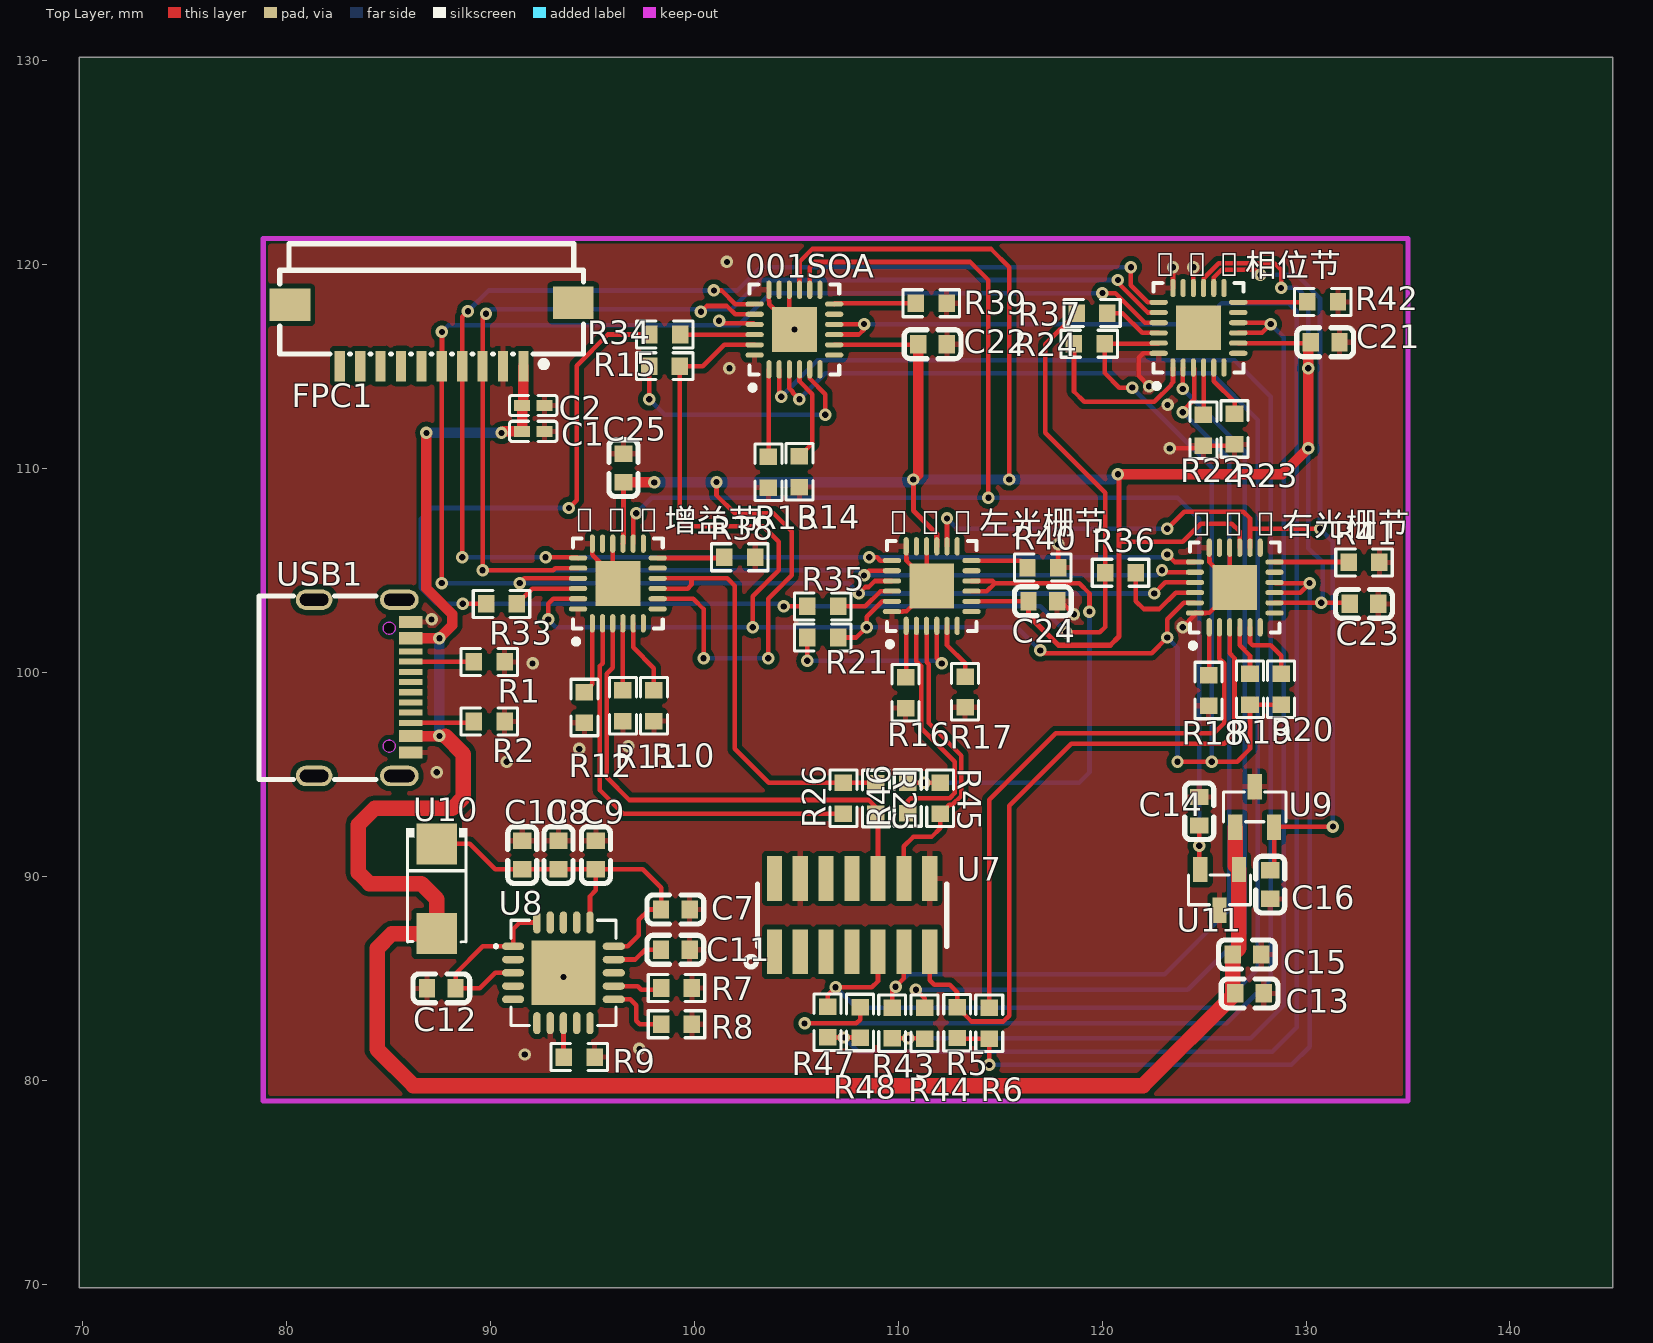
[diagram p0: Top Layer view]
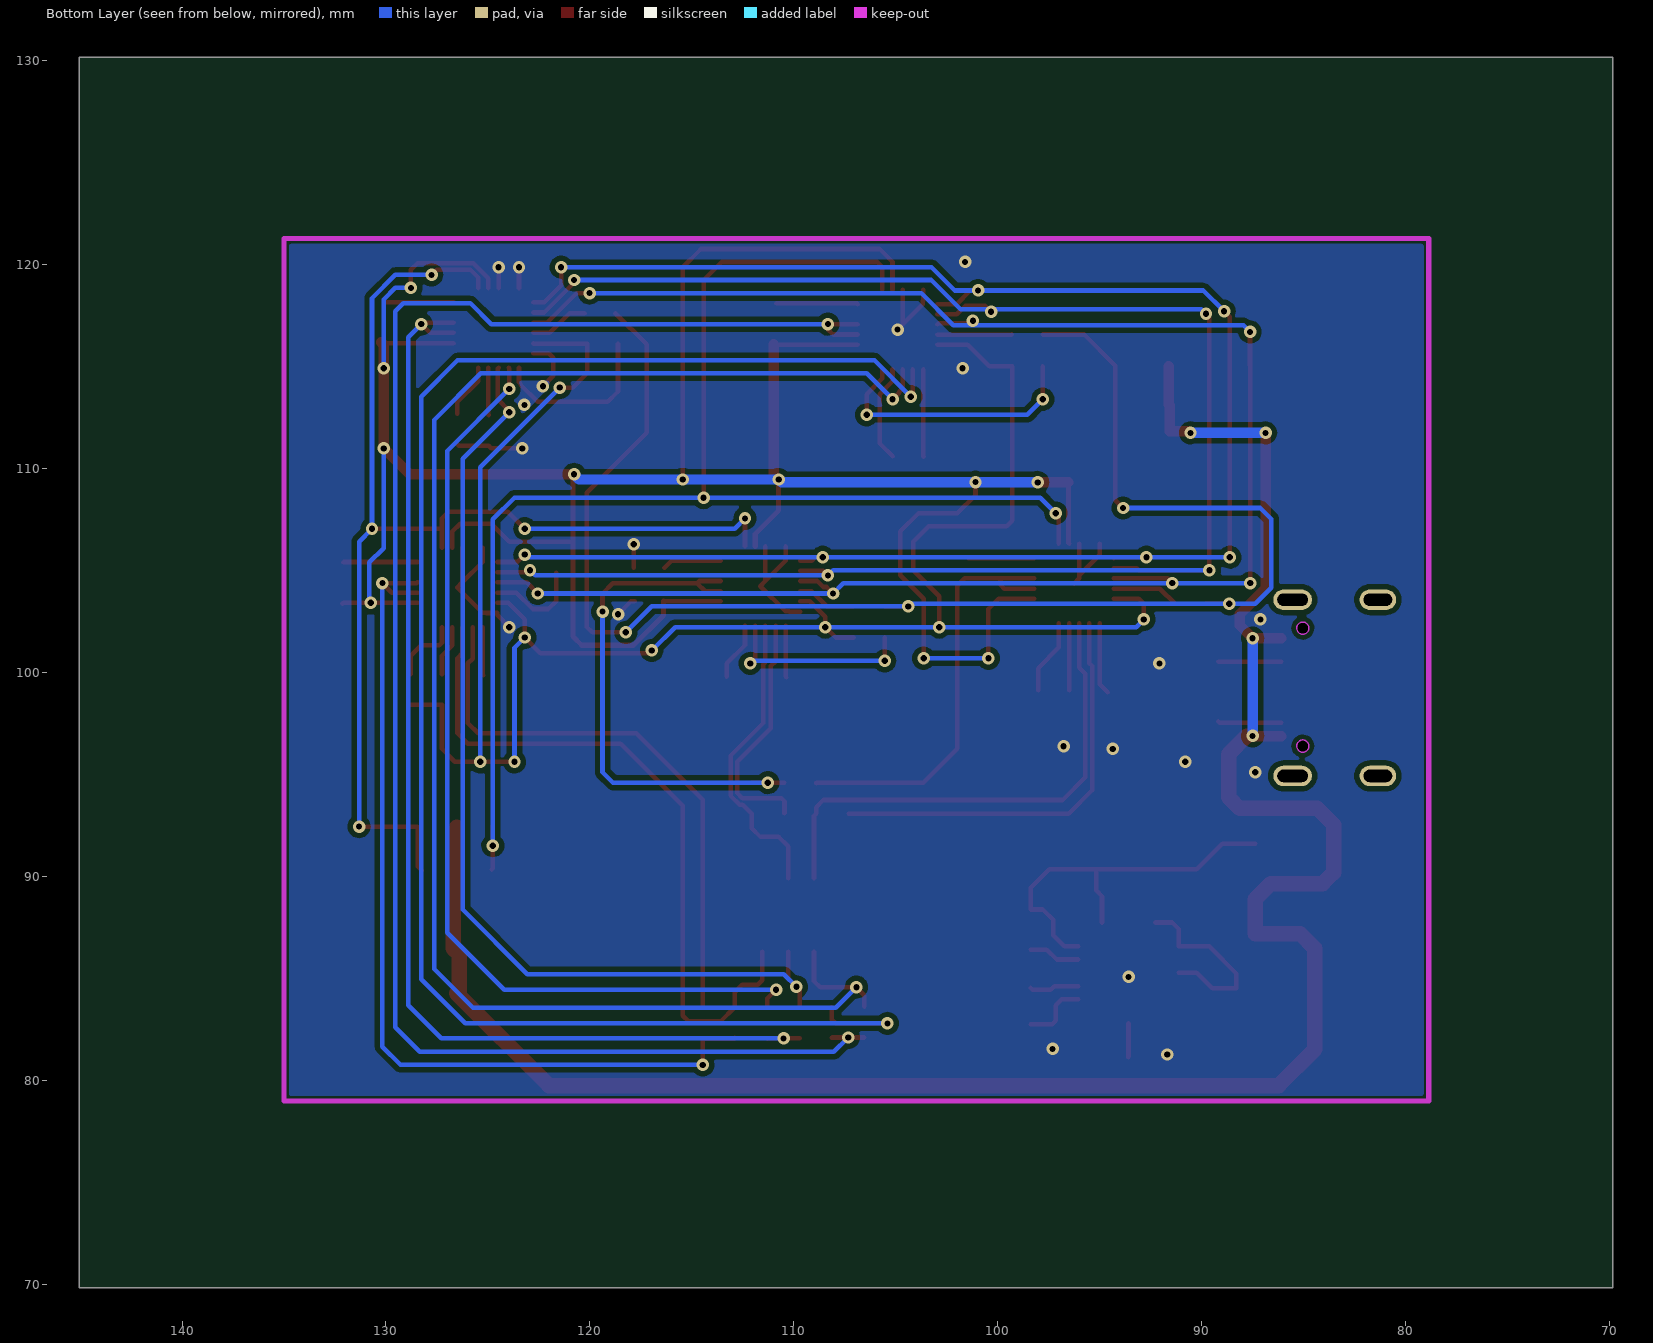
[diagram p1: Bottom Layer view, seen from below]
# Altium PCB MISC49874.pcbdoc
Units mm, origin at the board's own origin, x right, y up, seen from the top; angles counter-clockwise.
Board outline 75.18 x 60.32 mm, 2 copper layers (Top Layer, Bottom Layer), stack 1.58 mm thick; 69 components, 60 nets, 310 pads, 95 vias.

## Layer stack, top to bottom
Top Solder Mask Layer: solder mask 0.01, Dk 3.3
Top Layer: signal copper 0.035
Dielectric1: surface 1.51, FR4, Dk 4.5
Bottom Layer: signal copper 0.035
Bottom Solder Mask Layer: solder mask 0.01, Dk 3.3

## Board outline
145.034,69.85 69.85,69.85 69.85,130.175 145.034,130.175

## Design rules (kind name [scope] priority, off if disabled: settings)
BoardOutlineClearance copperThickness2oz_1 [All] p2 off: genericclearance=0.203 ignorepadtopadclearanceinfootprint=FALSE except(0: Arc-SplitContinuation Track-SplitContinuation SMDPad-SplitContinuation THPad-SplitContinuation Via-SplitContinuation Fill-SplitContinuation Region-SplitContinuation Poly-SplitContinuation Text-SplitContinuation Hole-SplitContinuation; 0.152: Arc-CutoutEdge SMDPad-CutoutEdge THPad-CutoutEdge Via-CutoutEdge Fill-CutoutEdge Region-CutoutEdge Text-CutoutEdge; 0.176: Hole-OutlineEdge Hole-CutoutEdge; 0.254: Poly-OutlineEdge Poly-CutoutEdge; 0.3: Arc-OutlineEdge Track-OutlineEdge SMDPad-OutlineEdge THPad-OutlineEdge Via-OutlineEdge Fill-OutlineEdge Region-OutlineEdge Text-OutlineEdge Track-CutoutEdge)
BoardOutlineClearance copperThickness1oz_1 [All] p4: genericclearance=0.102 ignorepadtopadclearanceinfootprint=FALSE except(0: Arc-SplitContinuation Track-SplitContinuation SMDPad-SplitContinuation THPad-SplitContinuation Via-SplitContinuation Fill-SplitContinuation Region-SplitContinuation Poly-SplitContinuation Text-SplitContinuation Hole-SplitContinuation; 0.152: SMDPad-CutoutEdge THPad-CutoutEdge Via-CutoutEdge Fill-CutoutEdge Region-CutoutEdge Text-CutoutEdge; 0.176: Hole-OutlineEdge Hole-CutoutEdge; 0.254: Poly-OutlineEdge Poly-CutoutEdge; 0.3: Arc-OutlineEdge Track-OutlineEdge SMDPad-OutlineEdge THPad-OutlineEdge Via-OutlineEdge Fill-OutlineEdge Region-OutlineEdge Text-OutlineEdge Arc-CutoutEdge Track-CutoutEdge)
Clearance copperThickness2oz [All] p1 off: gap=0.203 ignorepadtopadclearanceinfootprint=FALSE except(0.152: SMDPad-Track SMDPad-SMDPad THPad-Track SMDPad-THPad THPad-THPad Track-Via SMDPad-Via THPad-Via Via-Via Fill-Track Region-Track Fill-SMDPad Region-SMDPad Fill-THPad Region-THPad Fill-Via Region-Via Fill-Fill Fill-Region Region-Region Arc-Track Arc-SMDPad Arc-THPad Arc-Via Fill-Arc Region-Arc Arc-Arc Text-Track SMDPad-Text Text-THPad Text-Via Fill-Text Region-Text Arc-Text Text-Text; 0.176: Hole-Track Hole-SMDPad Hole-THPad Hole-Via Fill-Hole Region-Hole Hole-Arc Hole-Text; 0.254: Poly-Track Poly-SMDPad Poly-THPad Poly-Via Poly-Fill Poly-Region Poly-Poly Poly-Arc Poly-Text Poly-Hole)
Clearance copperThickness1oz [All] p3: gap=0.102 ignorepadtopadclearanceinfootprint=FALSE except(0.152: SMDPad-Track SMDPad-SMDPad THPad-Track SMDPad-THPad THPad-THPad Track-Via SMDPad-Via THPad-Via Via-Via Fill-Track Region-Track Fill-SMDPad Region-SMDPad Fill-THPad Region-THPad Fill-Via Region-Via Fill-Fill Fill-Region Region-Region Arc-Track Arc-SMDPad Arc-THPad Arc-Via Fill-Arc Region-Arc Arc-Arc Text-Track SMDPad-Text Text-THPad Text-Via Fill-Text Region-Text Arc-Text Text-Text; 0.176: Hole-Track Hole-SMDPad Hole-THPad Hole-Via Fill-Hole Region-Hole Hole-Arc Hole-Text; 0.254: Poly-Track Poly-SMDPad Poly-THPad Poly-Via Poly-Fill Poly-Region Poly-Poly Poly-Arc Poly-Text Poly-Hole)
DiffPairsRouting differentialPair [All] p1: maxlimit=0.152 minlimit=0.152 mostfreqgap=0.152 toplayer_minwidth=0.127 toplayer_prefwidth=0.254 toplayer_maxwidth=2.54 toplayer_mingap=0.152 toplayer_prefgap=0.152 toplayer_maxgap=0.152 bottomlayer_minwidth=0.127 bottomlayer_prefwidth=0.254 bottomlayer_maxwidth=2.54 bottomlayer_mingap=0.152 bottomlayer_prefgap=0.152 bottomlayer_maxgap=0.152 maxuncoupledlength=0.254
HoleToHoleClearance otherClearance [All] p1: gap=0.3 allowstackedmicrovias=TRUE
Length netLength [All] p1: minlimit=0 maxlimit=0
MatchedLengths netLengthTolerance [All] p1: tolerance=25.4
PasteMaskExpansion pasteMaskExpansion [All] p1: expansion=0
PlaneConnect innerPlane [All] p1: planeconnectstyle=Relief reliefexpansion=0.508 reliefentries=4 reliefconductorwidth=0.254 reliefairgap=0.254
PolygonConnect copperRegion [(InNet('GND') OR InNet('IOUT4'))] p1: connectstyle=Relief reliefconductorwidth=0.254 reliefentries=4 polygonreliefangle="90 Angle" airgapwidth=0.254 via.connectstyle=Relief via.reliefconductorwidth=0.254 via.reliefentries=4 via.polygonreliefangle="90 Angle" via.airgapwidth=0.254
RoutingVias viaSize [All] p1: holewidth=0.305 width=0.61 viastyle="Through Hole" minholewidth=0.3 minwidth=0.5 maxholewidth=6.3 maxwidth=10
SolderMaskExpansion solderMaskExpansion [IsVia] p1: expansion=-25.4 istentingtop=TRUE
SolderMaskExpansion solderMaskExpansion [All] p2: expansion=0.051 istentingtop=FALSE
Width copperThickness2oz_2 [All] p1 off: maxlimit=2.54 minlimit=0.203 preferedwidth=0.254
Width copperThickness1oz_2 [All] p2: maxlimit=2.54 minlimit=0.127 preferedwidth=0.254

## Components (designator, comment, footprint, x,y, rotation, side; value= is the part's Value field where it differs from the comment)
000增益节 "ADN8810ACPZ" LFCSP-24_L4.0-W4.0-P0.50-BL-EP2.3 96.255,104.377 r0 top
001SOA "ADN8810ACPZ" LFCSP-24_L4.0-W4.0-P0.50-BL-EP2.3 104.913,116.829 r0 top
010左光栅节 "ADN8810ACPZ" LFCSP-24_L4.0-W4.0-P0.50-BL-EP2.3 111.644,104.25 r0 top
011右光栅节 "ADN8810ACPZ" LFCSP-24_L4.0-W4.0-P0.50-BL-EP2.3 126.503,104.179 r0 top
100相位节 "ADN8810ACPZ" LFCSP-24_L4.0-W4.0-P0.50-BL-EP2.3 124.725,116.914 r0 top
C1 "10uF" C0402 92.108,111.835 r180 top
C2 "100nF" C0402 92.108,113.105 r180 top
C7 "10uF" C0603 99.075,88.392 r0 top
C8 "10uF" C0603 93.345,91.059 r90 top
C9 "0.1uF" C0603 95.178,91.059 r270 top
C10 "0.1uF" C0603 91.567,91.059 r270 top
C11 "1uF" C0603 99.075,86.415 r180 top
C12 "10uF" C0603 87.598,84.525 r0 top
C13 "2.2uF" C0603 127.229,84.277 r0 top
C14 "2.2uF" C0603 124.762,93.206 r270 top
C15 "2.2uF" C0603 127.102,86.182 r0 top
C16 "2.2uF" C0603 128.245,89.611 r90 top
C21 "100nF" C0603 130.937,116.205 r0 top
C22 "100nF" C0603 111.687,116.109 r0 top
C23 "100nF" C0603 132.842,103.378 r0 top
C24 "100nF" C0603 117.094,103.505 r0 top
C25 "100nF" C0603 96.531,110.034 r90 top
FPC1 "Header1X10" FPC-SMD_10P-P1.00_C9900008955 87.122,116.586 r180 top
R1 "5.1K" R0603 89.949,100.532 r180 top
R2 "5.1K" R0603 89.949,97.611 r180 top
R5 "2.2" R0603 112.895,82.843 r90 top
R6 "2.2" R0603 114.466,82.812 r270 top
R7 "0" R0603 99.13,84.539 r0 top
R8 "0" R0603 99.13,82.763 r0 top
R9 "0" R0603 94.361,81.153 r0 top
R10 "10K" R0603 98.024,98.382 r90 top
R11 "10K" R0603 96.5,98.382 r90 top
R12 "10K" R0603 94.615,98.298 r90 top
R13 "10K" R0603 103.634,109.833 r90 top
R14 "10K" R0603 105.156,109.855 r90 top
R15 "10K" R0603 98.546,115.031 r180 top
R16 "10K" R0603 110.365,99.017 r90 top
R17 "10K" R0603 113.284,99.06 r90 top
R18 "10K" R0603 125.224,99.131 r90 top
R19 "10K" R0603 127.254,99.187 r90 top
R20 "10K" R0603 128.778,99.187 r90 top
R21 "10K" R0603 106.299,101.727 r180 top
R22 "10K" R0603 124.968,111.887 r90 top
R23 "10K" R0603 126.494,111.95 r90 top
R24 "10K" R0603 119.374,116.132 r180 top
R25 "1.37" R0603 108.906,93.835 r270 top
R26 "1.37" R0603 107.313,93.846 r90 top
R33 "10K" R0603 90.551,103.378 r180 top
R34 "10K" R0603 98.552,116.586 r180 top
R35 "10K" R0603 106.299,103.251 r180 top
R36 "10K" R0603 120.904,104.902 r180 top
R37 "10K" R0603 119.507,117.633 r180 top
R38 "10K" R0603 102.235,105.664 r0 top
R39 "10K" R0603 111.624,118.119 r0 top
R40 "10K" R0603 117.094,105.156 r0 top
R41 "10K" R0603 132.842,105.41 r0 top
R42 "10K" R0603 130.815,118.183 r0 top
R43 "2.2" R0603 109.707,82.822 r90 top
R44 "2.2" R0603 111.299,82.811 r270 top
R45 "2.2" R0603 112.061,93.845 r270 top
R46 "2.2" R0603 110.469,93.856 r90 top
R47 "1.37" R0603 106.541,82.869 r90 top
R48 "1.37" R0603 108.134,82.852 r270 top
U7 "ATLS7503" HDR-SMD_14P-P1.27-V-F-R2-C7-LS4.8 107.74,88.116 r0 top
U8 "TPS7A4701RGWR" VQFN-20_L5.0-W5.0-P0.65-TL-EP 93.588,85.287 r0 top
U9 "REF2930AIDBZT" SOT-23-3_L2.9-W1.3-P1.90-LS2.4-BR 127.483,93.421 r270 top
U10 "SS310 Schottky diode SMA" SMA_L4.3-W2.6-LS5.1-R-RD 87.376,89.408 r270 top
U11 "REF2940AIDBZT" SOT-23-3_L2.9-W1.3-P1.90-LS2.4-BR 125.759,89.352 r90 top
USB1 "Type-C-16P" USB-C-SMD_GT-USB-7010E 83.726,99.262 r270 top

## Footprints (in the part's own frame and the unit in brackets; to place one, negate y for a bottom-side part, rotate by r counter-clockwise, add the part's x,y. Pads: shape width x height; smd on the part's side, far side on the other; paste and mask are expansions set on the pad)
C0402 [mm]
  rect 0.79x0.54 smd paste-100 mask+0.051: 1(-0.545,0) 2(0.545,0)
  silkscreen extent -1.17,-0.5 1.17,0.5
C0603 [mm]
  rect 0.8x0.9 smd: 1(-0.7,0) 2(0.7,0)
  silkscreen extent -1.39,-0.71 1.39,0.71
FPC-SMD_10P-P1.00_C9900008955 [mm]
  rect 0.5x1.5 smd: 1(-4.5,1.55) 2(-3.5,1.55) 3(-2.5,1.55) 4(-1.5,1.55) 5(-0.5,1.55) 6(0.5,1.55) 7(1.5,1.55) 8(2.5,1.55) 9(3.5,1.55) 10(4.5,1.55)
  rect 2x1.6 smd: 11(6.95,-1.45) 12(-6.95,-1.55)
  silkscreen extent -7.45,-4.45 7.45,1.6
HDR-SMD_14P-P1.27-V-F-R2-C7-LS4.8 [mm]
  rect 0.74x2.2 smd: 1(-3.81,-1.8) 2(-3.81,1.8) 3(-2.54,-1.8) 4(-2.54,1.8) 5(-1.27,-1.8) 6(-1.27,1.8) 7(0,-1.8) 8(0,1.8) 9(1.27,-1.8) 10(1.27,1.8) 11(2.54,-1.8) 12(2.54,1.8) 13(3.81,-1.8) 14(3.81,1.8)
  silkscreen extent -5.21,-2.54 4.64,1.52
LFCSP-24_L4.0-W4.0-P0.50-BL-EP2.3 [mm]
  oval 0.25x0.9 smd paste-100 mask+0.05: 1(-1.25,-1.951) 2(-0.75,-1.951) 3(-0.25,-1.951) 4(0.25,-1.951) 5(0.75,-1.951) 6(1.25,-1.951) 13(1.25,1.951) 14(0.75,1.951) 15(0.25,1.951) 16(-0.25,1.951) 17(-0.75,1.951) 18(-1.25,1.951)
  oval 0.9x0.25 smd paste-100 mask+0.05: 7(1.951,-1.25) 8(1.951,-0.75) 9(1.951,-0.25) 10(1.951,0.25) 11(1.951,0.75) 12(1.951,1.25) 19(-1.951,1.25) 20(-1.951,0.75) 21(-1.951,0.25) 22(-1.951,-0.25) 23(-1.951,-0.75) 24(-1.951,-1.25)
  rect 2.2x2.2 smd paste-100 mask+0.05: 25(0,0)
  silkscreen extent -2.2,-2.98 2.2,2.2
R0603 [mm]
  rect 0.806x0.864 smd paste-100 mask+0.051: 1(-0.753,0) 2(0.753,0)
  silkscreen extent -1.39,-0.66 1.39,0.66
SMA_L4.3-W2.6-LS5.1-R-RD [mm]
  rect 2x2 smd: 1(2.2,0) 2(-2.2,0)
  silkscreen extent -2.98,-1.5 2.6,1.5
SOT-23-3_L2.9-W1.3-P1.90-LS2.4-BR [mm]
  rect 1.25x0.7 smd: 1(1,-0.95) 2(1,0.95) 3(-1,0)
  silkscreen extent -0.73,-1.53 0.73,1.53
USB-C-SMD_GT-USB-7010E [mm]
  oval 1x1.9 hole 0.6 slot 1.5 at 90 deg paste+0 mask+0.05: 1(-4.32,1.815) 2(4.32,1.815)
  oval 1x1.8 hole 0.6 slot 1.4 at 90 deg paste+0 mask+0.05: 3(4.32,-2.365) 4(-4.32,-2.365)
  rect 0.6x1.15 smd paste-100 mask+0.05: A1B12(-3.232,2.365) A4B9(-2.432,2.365) B1A12(3.168,2.365) B4A9(2.368,2.365)
  rect 0.3x1.15 smd paste-100 mask+0.05: A5(-1.282,2.365) A6(-0.282,2.365) A7(0.218,2.365) A8(1.218,2.365) B5(1.718,2.365) B6(0.718,2.365) B7(-0.782,2.365) B8(-1.782,2.365)
  Board Outline Layer circle w0.003: c2.858,1.315 r0.3
  Board Outline Layer circle w0.003: c-2.922,1.315 r0.3
  Board Outline Layer region: 2.858,1.615 2.988,1.585 3.093,1.502 3.15,1.382 3.15,1.248 3.093,1.128 2.988,1.045 2.858,1.015 2.858,1.015 2.728,1.045 2.623,1.128 2.566,1.248 2.566,1.382 2.623,1.502 2.728,1.585 2.858,1.615
  Board Outline Layer region: 2.858,1.615 2.93,1.606 2.997,1.581 3.057,1.54 3.105,1.485 3.139,1.421 3.156,1.351 3.156,1.279 3.139,1.209 3.105,1.145 3.057,1.09 2.997,1.049 2.93,1.024 2.858,1.015 2.786,1.024 2.719,1.049 2.659,1.09 2.611,1.145 2.578,1.209 2.56,1.279 2.56,1.351 2.578,1.421 2.611,1.485 2.659,1.54 2.719,1.581 2.786,1.606
  Board Outline Layer region: -2.922,1.615 -2.792,1.585 -2.687,1.502 -2.63,1.382 -2.63,1.248 -2.687,1.128 -2.792,1.045 -2.922,1.015 -2.922,1.015 -3.052,1.045 -3.157,1.128 -3.214,1.248 -3.214,1.382 -3.157,1.502 -3.052,1.585 -2.922,1.615
  Board Outline Layer region: -2.922,1.615 -2.85,1.606 -2.783,1.581 -2.723,1.54 -2.675,1.485 -2.642,1.421 -2.624,1.351 -2.624,1.279 -2.642,1.209 -2.675,1.145 -2.723,1.09 -2.783,1.049 -2.85,1.024 -2.922,1.015 -2.994,1.024 -3.061,1.049 -3.121,1.09 -3.169,1.145 -3.203,1.209 -3.22,1.279 -3.22,1.351 -3.203,1.421 -3.169,1.485 -3.121,1.54 -3.061,1.581 -2.994,1.606
  Multi-Layer board cut-out: 2.858,1.615 2.988,1.585 3.093,1.502 3.15,1.382 3.15,1.248 3.093,1.128 2.988,1.045 2.858,1.015 2.858,1.015 2.728,1.045 2.623,1.128 2.566,1.248 2.566,1.382 2.623,1.502 2.728,1.585 2.858,1.615
  Multi-Layer board cut-out: -2.922,1.615 -2.792,1.585 -2.687,1.502 -2.63,1.382 -2.63,1.248 -2.687,1.128 -2.792,1.045 -2.922,1.015 -2.922,1.015 -3.052,1.045 -3.157,1.128 -3.214,1.248 -3.214,1.382 -3.157,1.502 -3.052,1.585 -2.922,1.615
  silkscreen extent -4.5,-5.07 4.5,0.66
VQFN-20_L5.0-W5.0-P0.65-TL-EP [mm]
  oval 1.087x0.364 smd paste-100 mask+0.051: 1(-2.468,1.3) 2(-2.468,0.65) 3(-2.468,0) 4(-2.468,-0.65) 5(-2.468,-1.3) 11(2.468,-1.3) 12(2.468,-0.65) 13(2.468,0) 14(2.468,0.65) 15(2.468,1.3)
  oval 0.364x1.087 smd paste-100 mask+0.051: 6(-1.3,-2.468) 7(-0.65,-2.468) 8(0,-2.468) 9(0.65,-2.468) 10(1.3,-2.468) 16(1.3,2.468) 17(0.65,2.468) 18(0,2.468) 19(-0.65,2.468) 20(-1.3,2.468)
  rect 3.15x3.15 smd paste-100 mask+0.051: 21(0,0)
  silkscreen extent -3.39,-2.58 2.58,2.58

## Via types
v1: diameter 0.61, hole 0.305, Top Layer to Bottom Layer, 95 vias

## Nets (pads, with @x,y where several pads share a name; then routed paths per layer and width w, separated by ;. In a path a pad name is that pad's centre, name@x,y a point inside that pad or via, vN(x,y) a via of type N, cw(c..) or ccw(c..) an arc to the next point about the centre after c; other vN are vias at no path point)
3.3V_ANA: 000增益节.8 000增益节.15 001SOA.8 001SOA.15 010左光栅节.8 010左光栅节.15 011右光栅节.8 011右光栅节.15 100相位节.8 100相位节.15 C21.1 C22.1 C23.1 C24.1 C25.1 | length 149.2
  Top Layer w0.225: 000增益节.15 96.531,106.354 C25.1 ; 000增益节.8 99.954,103.627 100.457,103.124 v1(100.457,100.711) ; v1(101.092,109.347) 101.092,108.712 101.981,107.823 103.886,107.823 104.775,106.934 104.775,104.775 103.632,103.632 v1(103.632,100.711) ; 001SOA.15 105.163,120.149 105.791,120.777 114.554,120.777 115.443,119.888 v1(115.443,109.474) ; 001SOA.8 110.957,116.078 C22.1 ; 010左光栅节.8 113.6,103.505 C24.1 ; 120.833,106.401 120.858,106.426 123.952,106.426 124.841,107.315 126.365,107.315 126.753,106.927 011右光栅节.15 ; 100相位节.15 124.975,119.342 125.722,120.088 128.451,120.088 128.778,119.761 v1(128.778,118.872) ; 100相位节.8 C21.1@130.195,116.163 ; 011右光栅节.8 v1(130.745,103.428) 132.092,103.428 C23.1
  Top Layer w0.254: v1(110.744,109.474) 110.744,107.95 111.894,106.8 010左光栅节.15 ; C24.1 116.394,102.808 117.856,101.346 120.396,101.346 120.833,101.783 120.833,106.401 v1@120.833,109.728
  Top Layer w0.508: C25.1 v1(98.044,109.334) ; v1(110.744,109.474) 110.987,109.717 C22.1 ; v1(120.777,109.728) 120.833,109.728 128.843,109.728 v1(130.113,110.998) 130.113,116.082 130.195,116.163 C21.1
  Bottom Layer w0.225: v1(100.457,100.711) v1(103.632,100.711) ; v1(128.778,118.872) 129.54,118.872 130.11,118.302 v1(130.11,114.935) ; v1(130.113,110.998) 130.113,106.107 130.81,105.41 130.81,103.494 v1(130.745,103.428)
  Bottom Layer w0.508: v1(98.044,109.334) 110.604,109.334 v1(110.744,109.474) v1(115.443,109.474) 120.523,109.474 v1(120.777,109.728)
3V3_OUT: 000增益节.23 001SOA.23 010左光栅节.23 011右光栅节.23 100相位节.23 R15.1 R19.1 R20.1 R21.1 R24.1 | length 101.1
  Top Layer w0.225: v1(92.837,102.616) 92.837,103.378 93.091,103.632 94.299,103.632 000增益节.23 ; v1(102.87,102.235) 102.87,103.759 104.14,105.029 104.14,106.426 103.378,107.188 99.568,107.188 99.299,107.457 R15.1 100.426,115.031 101.473,116.078 001SOA.23 ; R21.1 107.95,101.727 v1(108.458,102.235) 108.458,102.743 109.215,103.5 010左光栅节.23 ; v1(116.967,101.092) 117.094,100.965 122.428,100.965 v1(123.19,101.727) 123.19,102.616 124.002,103.428 011右光栅节.23 ; v1(121.475,113.983) 120.84,113.983 120.127,114.696 R24.1 122.744,116.132 100相位节.23 ; v1(123.698,95.631) v1(125.379,95.631) 126.619,95.631 127.254,96.266 R19.1 R20.1
  Bottom Layer w0.225: v1(92.837,102.616) 93.218,102.235 v1(102.87,102.235) v1(108.458,102.235) 115.824,102.235 v1(116.967,101.092) ; v1(121.475,113.983) 125.379,110.079 v1(125.379,95.631) ; v1(123.19,101.727) 123.698,101.219 v1(123.698,95.631)
5V_STABLE: U8.13
$1N135: 000增益节.12 R38.1 | length 3.3
  Top Layer w0.225: 000增益节.12 101.444,105.627 R38.1
$1N144: 000增益节.5 R10.2 | length 3.7
  Top Layer w0.225: 000增益节.5 97.005,101.242 98.024,100.223 R10.2
$1N147: 000增益节.22 R33.1 | length 3.3
  Top Layer w0.225: R33.1 92.053,104.127 000增益节.22
$1N160: 001SOA.5 R15.2 | length 13.1
  Top Layer w0.225: v1(97.792,113.411) R15.2 ; 001SOA.5 105.663,114.428 106.426,113.665 v1(106.426,112.649)
  Bottom Layer w0.225: v1(97.792,113.411) 98.554,112.649 v1(106.426,112.649)
$1N162: 001SOA.12 R39.1 | length 4
  Top Layer w0.225: 001SOA.12 106.904,118.119 R39.1
$1N163: 001SOA.22 R34.1 | length 3.7
  Top Layer w0.225: R34.1 99.313,116.579 001SOA.22
$1N165: 010左光栅节.12 R40.1 | length 2.9
  Top Layer w0.225: 010左光栅节.12 115.997,105.5 R40.1
$1N175: 010左光栅节.22 R35.1 | length 3
  Top Layer w0.225: R35.1 108.387,103.251 109.136,104 010左光栅节.22
$1N177: 010左光栅节.5 R17.2 | length 2.9
  Top Layer w0.225: 010左光栅节.5 112.394,101.347 113.284,100.457 R17.2
$1N190: 011右光栅节.12 R41.1 | length 3.6
  Top Layer w0.225: 011右光栅节.12 132.07,105.428 R41.1
$1N191: 011右光栅节.22 R36.1 | length 4.8
  Top Layer w0.225: R36.1 121.657,103.514 122.047,103.124 122.809,103.124 123.603,103.918 124.542,103.918 011右光栅节.22
$1N192: 011右光栅节.5 R20.2 | length 3.4
  Top Layer w0.225: 011右光栅节.5 127.253,101.474 127.381,101.346 128.27,101.346 128.778,100.838 R20.2
$1N195: 100相位节.12 R42.1 | length 3.4
  Top Layer w0.225: 100相位节.12 130.042,118.163 R42.1
$1N203: 100相位节.5 R23.2 | length 2.7
  Top Layer w0.225: 100相位节.5 125.475,114.301 126.494,113.282 R23.2
$1N206: 100相位节.22 R37.1 | length 2.9
  Top Layer w0.225: R37.1 121,117.633 121.969,116.664 100相位节.22
$1N212: C7.1 C8.1 C9.2 C10.2 U8.15 U8.16 U10.2 | length 19.2
  Top Layer w0.225: U10.2 88.986,91.608 90.235,90.359 C10.2 C8.1 C9.2 ; U8.16 94.888,89.046 95.178,89.336 C9.2 ; U8.15 96.747,86.587 97.282,87.122 97.282,87.884 97.79,88.392 C7.1 98.375,89.458 97.474,90.359 C9.2
$1N215: C12.2 U8.1 U8.3 U8.20 | length 9.4
  Top Layer w0.225: U8.3 90.24,85.287 89.478,84.525 C12.2 88.298,85.25 89.635,86.587 U8.1 91.119,87.436 91.438,87.755 U8.20
$1N217: R9.1 U8.8 | length 1.7
  Top Layer w0.225: U8.8 93.588,81.173 R9.1
$1N219: R7.1 U8.12 | length 2.4
  Top Layer w0.225: U8.12 97.227,84.637 97.409,84.455 98.293,84.455 R7.1
$1N220: R8.1 U8.11 | length 3.3
  Top Layer w0.225: U8.11 96.861,83.987 97.155,83.693 97.155,82.931 97.323,82.763 R8.1
$1N222: C11.2 U8.14 | length 2.5
  Top Layer w0.225: U8.14 97.113,85.937 97.591,86.415 C11.2
$1N225: 000增益节.1 R12.2 | length 3.5
  Top Layer w0.225: R12.2 95.005,99.442 000增益节.1
$1N226: 000增益节.4 R11.2 | length 3.3
  Top Layer w0.225: R11.2 96.505,99.14 000增益节.4
$1N227: 001SOA.1 R13.2 | length 4.3
  Top Layer w0.225: R13.2 103.663,110.616 001SOA.1
$1N228: 001SOA.4 R14.2 | length 4.8
  Top Layer w0.225: R14.2 105.791,111.243 105.791,113.665 105.163,114.293 001SOA.4
$1N231: 010左光栅节.1 R16.2 | length 2.5
  Top Layer w0.225: R16.2 110.394,99.8 010左光栅节.1
$1N233: 010左光栅节.4 R21.2 | length 9.7
  Top Layer w0.225: v1(105.546,100.584) R21.2 ; 010左光栅节.4 111.894,100.704 v1(112.141,100.457)
  Bottom Layer w0.225: v1(105.546,100.584) 112.014,100.584 v1(112.141,100.457)
$1N234: 011右光栅节.1 R18.2 | length 2.4
  Top Layer w0.225: R18.2 125.253,99.914 011右光栅节.1
$1N236: 011右光栅节.4 R19.2 | length 2.5
  Top Layer w0.225: 011右光栅节.4 126.753,101.339 127.254,100.838 R19.2
$1N240: 100相位节.4 R22.2 | length 2.3
  Top Layer w0.225: R22.2 124.975,112.647 100相位节.4
$1N242: 100相位节.1 R24.2 | length 8.5
  Top Layer w0.225: R24.2 118.62,113.79 119.126,113.284 122.555,113.284 123.382,114.111 123.382,114.155 123.475,114.248 100相位节.1
$1N278: U7.5
$1N324: R1.2 USB1.A5 | length 3.1
  Top Layer w0.225: USB1.A5 89.184,100.544 R1.2
$1N326: R2.2 USB1.B5 | length 3.1
  Top Layer w0.225: USB1.B5 89.129,97.544 R2.2
+5V_IN: C1.2 C2.2 C13.1 C15.1 FPC1.1 U9.1 U10.1 U11.1 USB1.A4B9 USB1.B4A9 | length 105.2
  Top Layer w0.508: USB1.B4A9 87.496,96.894 v1(87.503,96.901) ; USB1.A4B9 v1(87.503,101.694) 88.138,102.329 88.138,102.87 86.868,104.14 v1(86.868,111.76) ; v1(90.551,111.76) 90.626,111.835 C1.2 C2.2 91.622,113.163 FPC1.1
  Top Layer w0.762: v1@87.795,96.894 88.677,96.012 88.677,93.884 88.138,93.345 84.328,93.345 83.535,92.552 83.535,90.201 84.074,89.662 86.614,89.662 87.376,88.9 U10.1 85.176,87.208 84.455,86.487 84.455,81.534 86.233,79.756 122.008,79.756 C13.1 126.402,84.404 C15.1 126.709,86.489 U11.1 126.533,90.528 U9.1
  Bottom Layer w0.508: v1(86.868,111.76) v1(90.551,111.76) ; v1(87.503,96.901) v1(87.503,101.694)
ADN_CS_LASER: 000增益节.21 001SOA.21 010左光栅节.21 011右光栅节.21 100相位节.21 FPC1.5 | length 92.9
  Top Layer w0.225: v1(87.622,104.394) FPC1.5 87.63,115.044 v1(87.63,116.713) ; v1(91.44,104.394) 91.673,104.627 000增益节.21 ; v1(101.219,117.258) 101.34,117.136 102.905,117.136 001SOA.21 ; v1(108.077,103.886) 108.396,104.205 108.567,104.205 108.861,104.5 010左光栅节.21 ; v1(120.015,118.618) 120.65,118.618 122.104,117.164 100相位节.21 ; v1(122.555,103.886) 123.098,104.429 011右光栅节.21
  Bottom Layer w0.225: v1(87.622,104.394) v1(91.44,104.394) 107.569,104.394 v1(108.077,103.886) v1(122.555,103.886) ; v1(87.63,116.713) 87.949,117.032 102.173,117.032 103.759,118.618 v1(120.015,118.618)
ADN_SPI1_MOSI: 000增益节.19 001SOA.19 010左光栅节.19 011右光栅节.19 100相位节.19 FPC1.4 | length 89.4
  Top Layer w0.225: v1(88.622,105.664) FPC1.4 88.622,117.451 v1(88.9,117.729) ; v1(92.71,105.664) 94.267,105.664 000增益节.19 ; v1(100.965,118.745) 101.346,118.745 102.013,118.078 001SOA.19 ; v1(108.585,105.664) 108.966,105.664 109.13,105.5 010左光栅节.19 ; v1(121.412,119.888) 121.412,118.999 122.248,118.163 100相位节.19 ; v1(123.19,105.791) 123.553,105.428 011右光栅节.19
  Bottom Layer w0.225: v1(88.622,105.664) v1(92.71,105.664) v1(108.585,105.664) 123.063,105.664 v1(123.19,105.791) ; v1(88.9,117.729) 89.916,118.745 v1(100.965,118.745) 102.108,118.745 103.251,119.888 v1(121.412,119.888)
ADN_SPI1_SCK: 000增益节.20 001SOA.20 010左光栅节.20 011右光栅节.20 100相位节.20 FPC1.3 | length 91.3
  Top Layer w0.225: v1(89.789,117.602) 89.622,117.435 FPC1.3 v1(89.622,105.029) 93.078,105.029 93.176,105.127 000增益节.20 ; v1(100.33,117.706) 100.607,117.983 101.6,117.983 102.004,117.579 001SOA.20 ; v1(108.331,104.775) 108.556,105 010左光栅节.20 ; v1(120.777,119.257) 120.777,119.126 122.239,117.664 100相位节.20 ; v1(122.936,105.029) 123.036,104.929 011右光栅节.20
  Bottom Layer w0.225: v1(89.622,105.029) 108.077,105.029 v1(108.331,104.775) 122.682,104.775 v1(122.936,105.029) ; v1(89.789,117.602) 90.014,117.827 101.825,117.827 103.255,119.257 v1(120.777,119.257)
FB1: 000增益节.3 R25.2 U7.10 | length 25
  Top Layer w0.225: 000增益节.3 96.005,100.25 95.704,99.949 95.704,94.869 96.813,93.76 108.551,93.76 108.906,93.405 R25.2 109.01,92.977 U7.10
FB2: 001SOA.3 R47.2 U7.9 | length 79.2
  Top Layer w0.225: 001SOA.3 104.663,113.947 104.837,113.774 104.837,113.73 v1(105.156,113.411) ; R47.2 106.541,84.189 v1(106.934,84.582) 108.712,84.582 109.01,84.88 U7.9
  Bottom Layer w0.225: v1(105.156,113.411) 106.426,114.681 125.349,114.681 127.635,112.395 127.635,85.471 125.73,83.566 107.95,83.566 v1(106.934,84.582)
FB3: 010左光栅节.3 R45.2 U7.12 | length 14.9
  Top Layer w0.225: U7.12 110.28,91.484 110.744,91.948 111.633,91.948 112.061,92.376 R45.2 112.495,93.526 112.66,93.526 113.103,93.969 113.103,95.939 111.506,97.536 111.506,100.411 111.394,100.524 010左光栅节.3
FB4: 011右光栅节.3 R5.2 U7.13 | length 34.8
  Top Layer w0.225: U7.13 111.55,84.919 111.76,84.709 112.522,84.709 112.895,84.336 R5.2 113.594,82.897 115.155,82.897 115.443,83.185 115.443,93.472 118.491,96.52 125.984,96.52 126.492,97.028 126.492,100.711 126.253,100.95 011右光栅节.3
FB5: 100相位节.3 R43.2 U7.11 | length 48.7
  Top Layer w0.225: R43.2 109.707,84.434 110.28,85.007 U7.11 ; v1(123.952,112.776) 123.952,112.834 124.522,113.403 124.522,114.916 100相位节.3
  Bottom Layer w0.225: v1(109.871,84.598) 110.49,85.217 123.063,85.217 126.238,88.392 126.238,110.49 v1(123.952,112.776)
GND: 000增益节.16 000增益节.18 000增益节.24 000增益节.25 001SOA.16 001SOA.18 001SOA.24 001SOA.25 010左光栅节.16 010左光栅节.18 010左光栅节.24 010左光栅节.25 011右光栅节.16 011右光栅节.18 011右光栅节.24 011右光栅节.25 100相位节.16 100相位节.18 100相位节.24 C1.1 C2.1 C7.2 C8.2 C9.1 C10.1 C11.1 C12.1 C13.2 C14.1 C15.2 C16.1 C21.2 C22.2 C23.2 C24.2 C25.2 FPC1.2 R1.1 R2.1 R7.2 R8.2 R9.2 R10.1 R11.1 R12.1 R13.1 R14.1 R16.1 R17.1 R18.1 R22.1 R23.1 R38.2 R39.2 R40.2 R41.2 R42.2 U7.4 U7.14 U8.7 U8.21 U9.3 U11.3 USB1.A1B12 USB1.B1A12 | length 32.6
  Top Layer w0.225: 000增益节.18 95.005,105.801 95.019,105.788 95.019,105.768 000增益节.25@96.005,104.782 ; 000增益节.16 000增益节.25@96.005,104.782 ; 000增益节.25 96.005,104.627 000增益节.25@96.005,104.782 ; 001SOA.18 103.663,118.253 103.677,118.24 103.677,118.065 001SOA.25@104.663,117.079 ; 001SOA.16 001SOA.25@104.663,117.079 ; v1(104.913,116.829) 001SOA.25@104.663,117.079 ; 010左光栅节.24 110.22,103 110.233,103.014 110.408,103.014 010左光栅节.25 010左光栅节.25@111.394,104.5 ; 010左光栅节.18 110.394,105.674 110.408,105.661 110.408,105.486 010左光栅节.25@111.394,104.5 ; 010左光栅节.16 010左光栅节.25@111.394,104.5 ; C24.2 117.983,103.505 v1(118.618,102.87) ; R40.2 v1(117.847,106.299) ; v1(122.301,114.046) 121.793,114.554 121.793,115.443 122.014,115.664 100相位节.24 ; v1(123.317,110.998) 124.832,110.998 R22.1 126.431,111.134 R23.1 ; 100相位节.18 v1(123.475,119.888) ; v1(123.952,102.235) 124.552,102.835 011右光栅节.24 125.079,102.929 125.092,102.942 125.267,102.942 011右光栅节.25 011右光栅节.25@126.253,104.429 ; 100相位节.16 v1(124.475,119.888) ; 011右光栅节.18 125.253,105.603 125.267,105.59 125.267,105.415 011右光栅节.25@126.253,104.429 ; 011右光栅节.16 011右光栅节.25@126.253,104.429
  other v1: 91.694,81.28 97.312,81.553 93.588,85.082 87.376,95.123 90.805,95.631 94.361,96.266 96.774,96.393 92.075,100.457 87.122,102.616 123.212,113.135 101.727,114.935 101.6,120.142
IOUT1: 000增益节.9 000增益节.10 R25.1 R26.2 | length 21.6
  Top Layer w0.225: 000增益节.9 99.682,104.127 99.867,104.312 99.867,104.627 ; 000增益节.10 99.867,104.627 ; R25.1 108.895,94.599 R26.2 103.648,94.599 101.981,96.266 101.981,104.267 101.621,104.627 99.867,104.627
IOUT2: 001SOA.9 001SOA.10 R47.1 R48.2 | length 84.8
  Top Layer w0.225: R47.1 v1(107.33,82.116) 108.117,82.116 R48.2 ; 001SOA.9 106.871,116.586 108.077,116.586 108.331,116.84 v1(108.331,117.094) 108.316,117.079 001SOA.10
  Bottom Layer w0.225: v1(107.33,82.116) 108.039,81.407 128.334,81.407 129.54,82.613 129.54,117.729 129.159,118.11 125.857,118.11 124.841,117.094 v1(108.331,117.094)
IOUT3: 010左光栅节.9 010左光栅节.10 R45.1 R46.2 | length 26
  Top Layer w0.225: R46.2 v1(111.274,94.61) 112.051,94.61 R45.1 ; 010左光栅节.9 114.352,104 114.746,104.394 ; 010左光栅节.10 114.64,104.5 114.746,104.394 ; v1(119.38,102.997) 119.38,103.886 118.872,104.394 114.746,104.394
  Bottom Layer w0.225: v1(111.274,94.61) 118.867,94.61 119.38,95.123 v1(119.38,102.997)
IOUT4: 011右光栅节.9 011右光栅节.10 R5.1 R6.2 | length 45.3
  Top Layer w0.225: R5.1 112.927,82.058 R6.2 v1(114.466,80.772) ; 011右光栅节.9 129.71,103.929 v1(130.175,104.394) 128.488,104.394 011右光栅节.10
  Bottom Layer w0.225: v1(114.466,80.772) 129.286,80.772 130.175,81.661 v1(130.175,104.394)
IOUT5: 100相位节.9 100相位节.10 R43.1 R44.2 | length 57.7
  Top Layer w0.225: R43.1 v1(110.502,82.068) 111.289,82.068 R44.2 ; 100相位节.9 127.84,116.664 v1(128.27,117.094) 128.2,117.164 100相位节.10
  Bottom Layer w0.225: v1(110.502,82.068) 127.28,82.068 128.905,83.693 128.905,116.459 v1(128.27,117.094)
RSN1: 000增益节.2 R26.1 | length 20.7
  Top Layer w0.225: 000增益节.2 95.505,100.458 95.377,100.33 95.377,94.234 96.518,93.093 R26.1
RSN2: 001SOA.2 R48.1 | length 82.6
  Top Layer w0.225: 001SOA.2 104.163,113.642 v1(104.267,113.538) ; v1(105.41,82.804) 107.95,82.804 108.134,82.988 R48.1
  Bottom Layer w0.225: v1(104.267,113.538) 106.045,115.316 126.492,115.316 128.27,113.538 128.27,84.963 126.111,82.804 v1(105.41,82.804)
RSN3: 010左光栅节.2 R46.1 | length 12.1
  Top Layer w0.225: R46.1 110.458,93.114 110.458,93.694 110.617,93.853 112.525,93.853 112.776,94.104 112.776,95.631 111.125,97.282 111.125,100.33 110.894,100.561 010左光栅节.2
RSN4: 011右光栅节.2 R6.1 | length 28.1
  Top Layer w0.225: R6.1 114.466,93.765 117.729,97.028 125.476,97.028 125.984,97.536 125.984,100.457 125.753,100.688 011右光栅节.2
RSN5: 100相位节.2 R44.1 | length 47.3
  Top Layer w0.225: v1(110.871,84.455) 111.299,84.027 R44.1 ; v1(123.952,113.919) 123.952,114.94 100相位节.2
  Bottom Layer w0.225: v1(110.871,84.455) 124.206,84.455 127,87.249 127,110.871 v1(123.952,113.919)
RST: R33.2 R34.2 R35.2 R36.2 R37.2 | length 76.3
  Top Layer w0.225: v1(88.646,103.378) R33.2 ; v1(93.853,108.077) 94.234,108.458 94.234,115.062 95.758,116.586 R34.2 ; v1(104.394,103.251) R35.2 ; v1(118.237,101.981) 119.888,101.981 120.151,102.244 R36.2 120.151,108.83 117.221,111.76 117.221,116.1 R37.2
  Bottom Layer w0.225: v1(93.853,108.077) 87.122,108.077 86.582,107.537 86.582,104.172 87.376,103.378 v1(88.646,103.378) 104.267,103.378 v1(104.394,103.251) 116.967,103.251 v1(118.237,101.981)
VREF_3V: 010左光栅节.14 011右光栅节.14 100相位节.14 C16.2 U9.2 | length 59.5
  Top Layer w0.225: 010左光栅节.14 v1(112.395,107.569) ; v1(123.19,107.061) 124.029,107.9 126.923,107.9 127.253,107.57 127.253,107.061 ; 100相位节.14 125.476,119.38 125.857,119.761 127.508,119.761 v1(127.762,119.507) ; 011右光栅节.14 127.253,107.061 ; C16.2 128.433,90.499 U9.2 128.468,92.456 v1(131.318,92.456) ; v1(130.683,107.061) 127.253,107.061
  Bottom Layer w0.225: v1(112.395,107.569) 112.903,107.061 v1(123.19,107.061) ; v1(127.762,119.507) 129.54,119.507 130.683,118.364 v1(130.683,107.061) 131.318,106.426 v1(131.318,92.456)
VREF_4.1V: 000增益节.14 001SOA.14 C14.2 U11.2 | length 69.1
  Top Layer w0.225: 000增益节.14 97.005,107.673 v1(97.155,107.823) ; 001SOA.14 105.663,119.887 105.918,120.142 113.538,120.142 114.427,119.253 v1(114.427,108.585) ; C14.2 v1(124.762,91.518) 124.762,90.399 U11.2
  Bottom Layer w0.225: v1(97.155,107.823) 97.917,108.585 v1(114.427,108.585) 123.698,108.585 124.762,107.521 v1(124.762,91.518)
pads on no net: 000增益节.6 000增益节.7 000增益节.11 000增益节.13 000增益节.17 001SOA.6 001SOA.7 001SOA.11 001SOA.13 001SOA.17 010左光栅节.6 010左光栅节.7 010左光栅节.11 010左光栅节.13 010左光栅节.17 011右光栅节.6 011右光栅节.7 011右光栅节.11 011右光栅节.13 011右光栅节.17 100相位节.6 100相位节.7 100相位节.11 100相位节.13 100相位节.17 100相位节.25 FPC1.6 FPC1.7 FPC1.8 FPC1.9 FPC1.10 FPC1.11 FPC1.12 U7.1 U7.2 U7.3 U7.6 U7.7 U7.8 U8.2 U8.4 U8.5 U8.6 U8.9 U8.10 U8.17 U8.18 U8.19 USB1.1 USB1.2 USB1.3 USB1.4 USB1.A6 USB1.A7 USB1.A8 USB1.B6 USB1.B7 USB1.B8

## Polygon pours and split planes (outlines as drawn)
GND on Top Layer (solid, remove dead copper, pour order 0): 76.2,123.825 76.2,76.2 136.906,76.2 136.906,123.825
GND on Bottom Layer (solid, remove dead copper, pour order 2): 76.962,123.571 76.962,76.962 138.684,76.962 138.684,123.571

## Keep-outs
Board Outline Layer:
  lines w0.254: 78.867,78.994 78.867,121.285 135.001,121.285 135.001,78.994 78.867,78.994